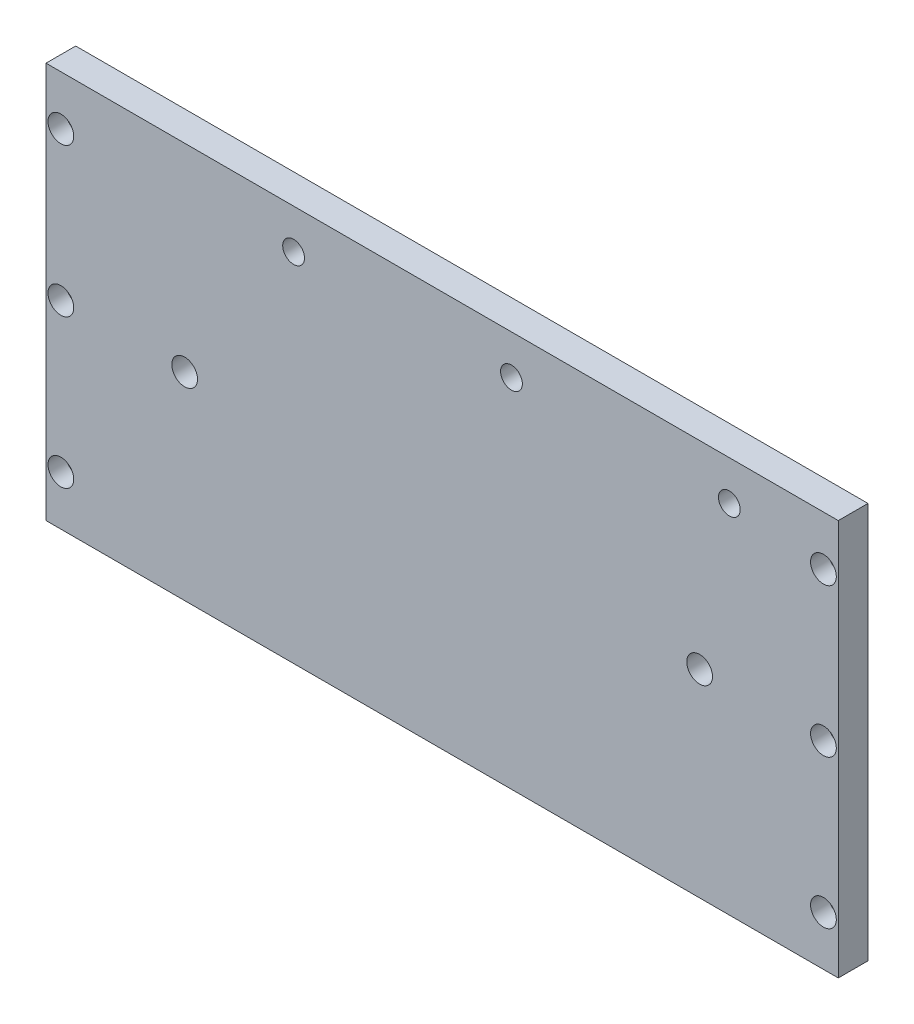
from build123d import *

# Parameters (mm, degrees)
SKETCH1_W               = 400
SKETCH1_H               = 200
BOSS_EXTRUDE1_DEPTH     = 15
SKETCH2_R               = 6.5
CUT_EXTRUDE1_DEPTH      = 9
LPATTERN1_COUNT         = 3
LPATTERN1_PITCH         = 75
MIRROR1_COPY_1_SKETCH_R = 6.5
MIRROR1_COPY_1_DEPTH    = 9
MIRROR1_COPY_2_SKETCH_R = 6.5
MIRROR1_COPY_2_DEPTH    = 9
SKETCH3_R               = 4.5
CUT_EXTRUDE2_DEPTH      = 85
LPATTERN2_COUNT         = 3
LPATTERN2_PITCH         = 75
MIRROR2_COPY_1_SKETCH_R = 4.5
MIRROR2_COPY_1_DEPTH    = 85
MIRROR2_COPY_2_SKETCH_R = 4.5
MIRROR2_COPY_2_DEPTH    = 85
SKETCH4_R               = 6.5
CUT_EXTRUDE3_DEPTH      = 85
LPATTERN3_COUNT         = 3
LPATTERN3_PITCH         = 130
SKETCH5_R               = 5.5
CUT_EXTRUDE4_DEPTH      = 51
LPATTERN4_COUNT         = 3
LPATTERN4_PITCH         = 110


with BuildPart() as part:
    # Sketch1 → Boss-Extrude1 (new body)
    with BuildSketch(Plane.XY):
        Rectangle(SKETCH1_W, SKETCH1_H)
    extrude(amount=BOSS_EXTRUDE1_DEPTH)

    # Sketch2 → Cut-Extrude1 (cut)
    with BuildSketch(Plane.XY.offset(15)):
        with Locations((-192.5, 75)):
            Circle(SKETCH2_R)
    cut_extrude1 = extrude(amount=-CUT_EXTRUDE1_DEPTH, mode=Mode.SUBTRACT)

    # LPattern1: Cut-Extrude1 ×3
    with Locations(*[(0, -i * LPATTERN1_PITCH, 0) for i in range(1, LPATTERN1_COUNT)]):
        add(cut_extrude1, mode=Mode.SUBTRACT)

    # Mirror1: Cut-Extrude1 across plane
    add(cut_extrude1.mirror(Plane(origin=(0, 0, 0), x_dir=(0, 0, 1), z_dir=(1, 0, 0))), mode=Mode.SUBTRACT)

    # Mirror1 copy 1 sketch → Mirror1 copy 1 (cut)
    with BuildSketch(Plane(origin=(0, -75, 15), x_dir=(-1, 0, 0), z_dir=(0, 0, 1))):
        with Locations((-192.5, -75)):
            Circle(MIRROR1_COPY_1_SKETCH_R)
    extrude(amount=-MIRROR1_COPY_1_DEPTH, mode=Mode.SUBTRACT)

    # Mirror1 copy 2 sketch → Mirror1 copy 2 (cut)
    with BuildSketch(Plane(origin=(0, -150, 15), x_dir=(-1, 0, 0), z_dir=(0, 0, 1))):
        with Locations((-192.5, -75)):
            Circle(MIRROR1_COPY_2_SKETCH_R)
    extrude(amount=-MIRROR1_COPY_2_DEPTH, mode=Mode.SUBTRACT)

    # Sketch3 → Cut-Extrude2 (cut)
    with BuildSketch(Plane.XY.offset(15)):
        with Locations((-192.5, 75)):
            Circle(SKETCH3_R)
    cut_extrude2 = extrude(amount=-CUT_EXTRUDE2_DEPTH, mode=Mode.SUBTRACT)

    # LPattern2: Cut-Extrude2 ×3
    with Locations(*[(0, -i * LPATTERN2_PITCH, 0) for i in range(1, LPATTERN2_COUNT)]):
        add(cut_extrude2, mode=Mode.SUBTRACT)

    # Mirror2: Cut-Extrude2 across plane
    add(cut_extrude2.mirror(Plane(origin=(0, 0, 0), x_dir=(0, 0, 1), z_dir=(1, 0, 0))), mode=Mode.SUBTRACT)

    # Mirror2 copy 1 sketch → Mirror2 copy 1 (cut)
    with BuildSketch(Plane(origin=(0, -75, 15), x_dir=(-1, 0, 0), z_dir=(0, 0, 1))):
        with Locations((-192.5, -75)):
            Circle(MIRROR2_COPY_1_SKETCH_R)
    extrude(amount=-MIRROR2_COPY_1_DEPTH, mode=Mode.SUBTRACT)

    # Mirror2 copy 2 sketch → Mirror2 copy 2 (cut)
    with BuildSketch(Plane(origin=(0, -150, 15), x_dir=(-1, 0, 0), z_dir=(0, 0, 1))):
        with Locations((-192.5, -75)):
            Circle(MIRROR2_COPY_2_SKETCH_R)
    extrude(amount=-MIRROR2_COPY_2_DEPTH, mode=Mode.SUBTRACT)

    # Sketch4 → Cut-Extrude3 (cut)
    with BuildSketch(Plane.XY.offset(15)):
        with Locations((-130, 0)):
            Circle(SKETCH4_R)
    cut_extrude3 = extrude(amount=-CUT_EXTRUDE3_DEPTH, mode=Mode.SUBTRACT)

    # LPattern3: Cut-Extrude3 ×3, 1 skipped
    with Locations(*[(i * LPATTERN3_PITCH, 0, 0) for i in range(1, LPATTERN3_COUNT) if i not in (1,)]):
        add(cut_extrude3, mode=Mode.SUBTRACT)

    # Sketch5 → Cut-Extrude4 (cut)
    with BuildSketch(Plane.XY.offset(15)):
        with Locations((-75, 80)):
            Circle(SKETCH5_R)
    cut_extrude4 = extrude(amount=-CUT_EXTRUDE4_DEPTH, mode=Mode.SUBTRACT)

    # LPattern4: Cut-Extrude4 ×3
    with Locations(*[(i * LPATTERN4_PITCH, 0, 0) for i in range(1, LPATTERN4_COUNT)]):
        add(cut_extrude4, mode=Mode.SUBTRACT)


solid = part.part
